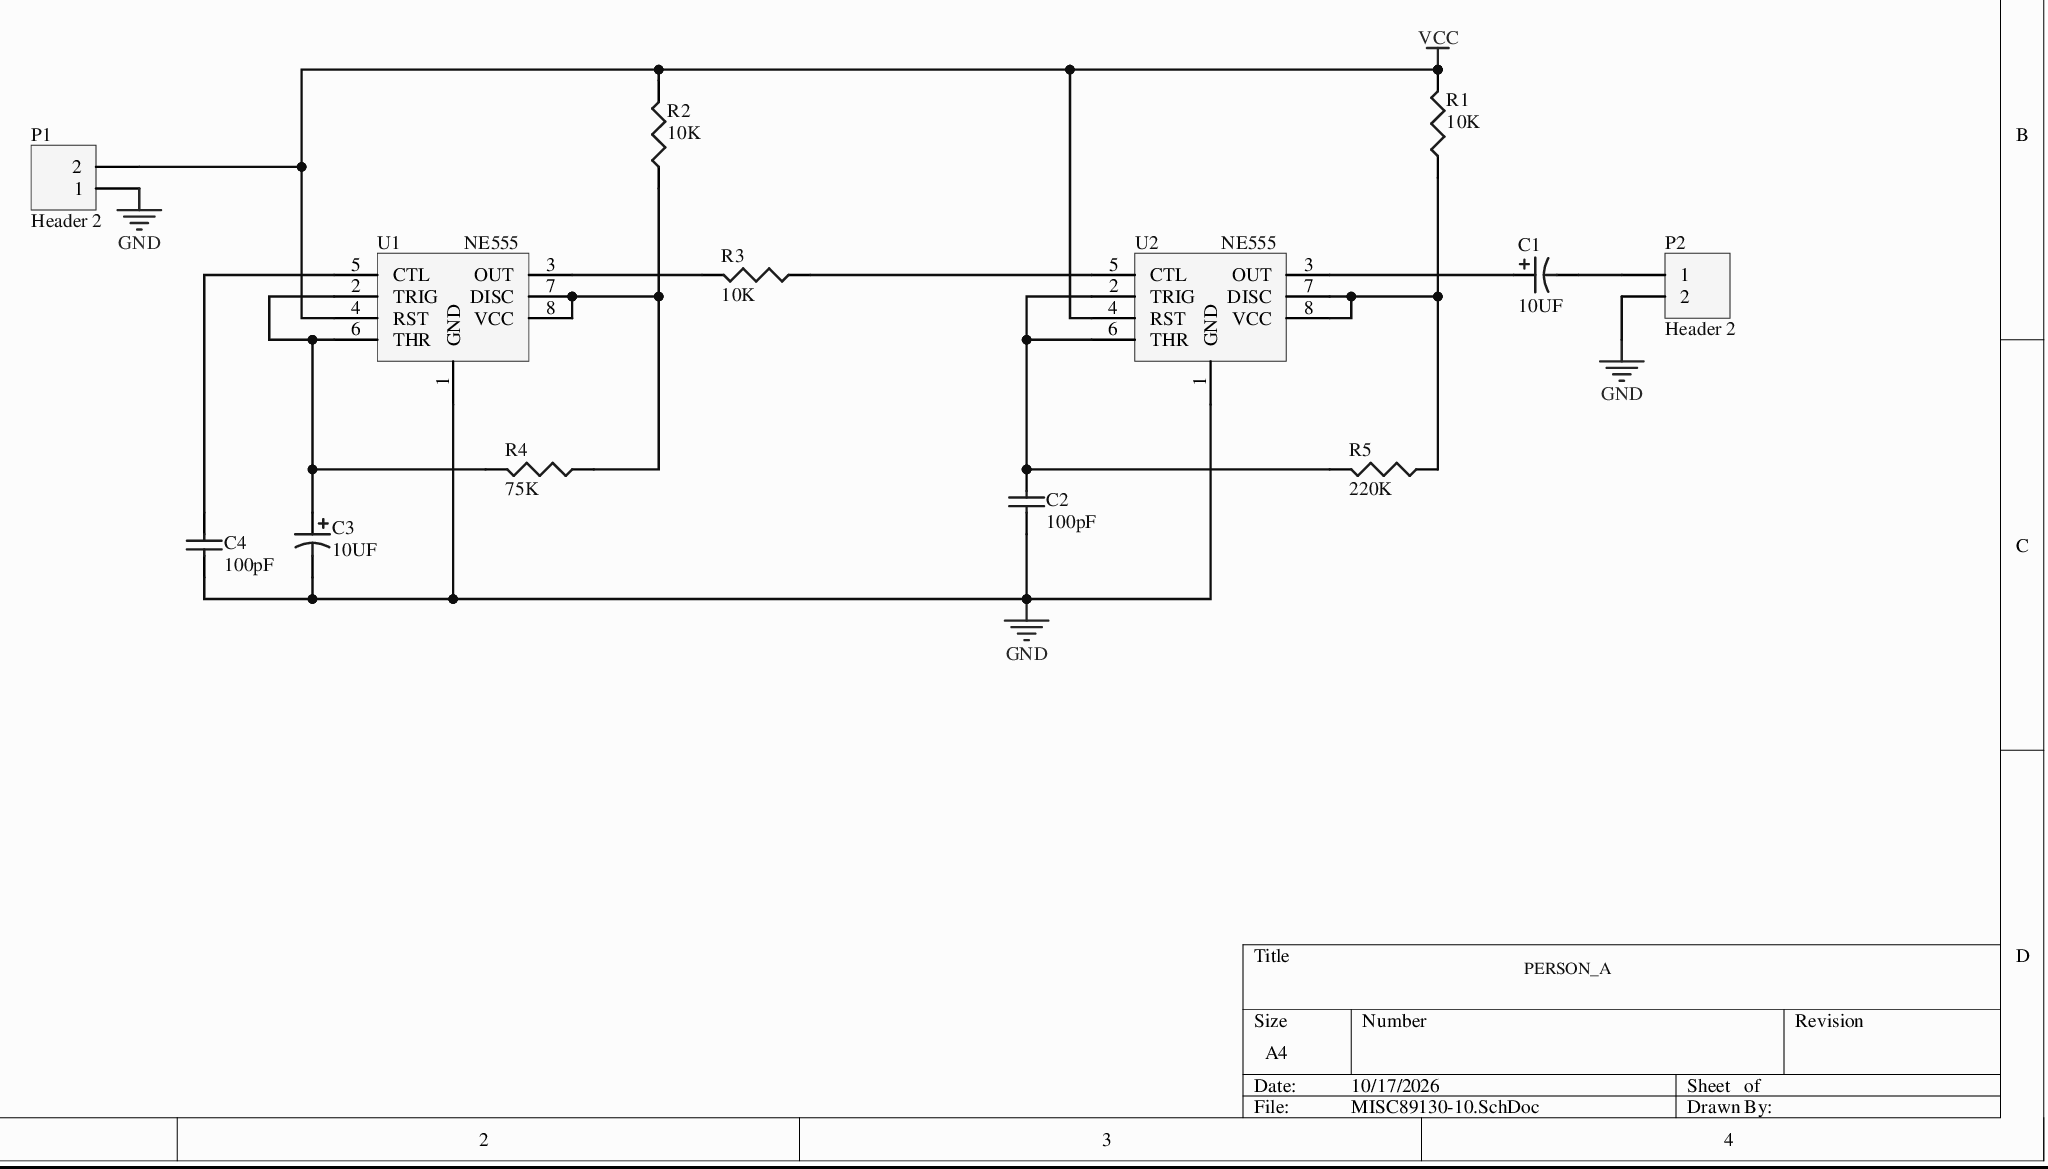
[diagram p0: MISC89130-10.SchDoc]
# Altium project MISC89130-7.PrjPcb
1 sheet, 13 parts. Net scope: global (net labels, ports and power ports of the same name join across sheets).
Board file: MISC89130.PcbDoc

## Sheet MISC89130-10.SchDoc
size A4

### Parts
C1  10UF  [C1206]
C2  value 100pF  [J1-0603]  (hidden comment: Cap)
C3  10UF  [C1206]
C4  value 100pF  [J1-0603]  (hidden comment: Cap)
P1  Header 2  [HDR1X2]
P2  Header 2  [HDR1X2]
R1  10K  [J1-0603]
R2  10K  [J1-0603]
R3  10K  [J1-0603]
R4  75K  [J1-0603]
R5  220K  [J1-0603]
U1  NE555  [DIP8]
U2  NE555  [DIP8]

### Nets
GND: C2.1 C3.2 C4.1 P1.1 P2.2 U1.1(GND) U2.1(GND)
VCC: P1.2 R1.2 R2.2 U1.4(RST) U2.4(RST)
NetC1_1: C1.1 U2.3(OUT)
NetC1_2: C1.2 P2.1
NetC2_2: C2.2 R5.2 U2.2(TRIG) U2.6(THR)
NetC3_1: C3.1 R4.2 U1.2(TRIG) U1.6(THR)
NetC4_2: C4.2 U1.5(CTL)
NetR1_1: R1.1 R5.1 U2.7(DISC) U2.8(VCC)
NetR2_1: R2.1 R4.1 U1.7(DISC) U1.8(VCC)
NetR3_1: R3.1 U2.5(CTL)
NetR3_2: R3.2 U1.3(OUT)

### Notes on the sheet
- PERSON_A

### Library data of the parts
C1 C3 = Cap Pol3: Polarized Capacitor (Surface Mount); Value: 100pF; Published: 8-Jun-2000; LatestRevisionDate: 29-May-2009; LatestRevisionNote: IPC-7351 Footprint Added.; PackageReference: C0805; PackageDescription: Chip Capacitor; Publisher: Altium Limited
C2 C4 = Cap: Capacitor; Published: 8-Jun-2000; LatestRevisionDate: 17-Jul-2002; LatestRevisionNote: Re-released for DXP Platform.; PackageReference: RAD-0.3; PackageDescription: Radial Cap, Thru-Hole; 2 Leads; 0.3 in Pin Spacing; Publisher: Altium Limited
P1 P2 = Header 2: Header, 2-Pin; LatestRevisionDate: 17-Jul-2002; LatestRevisionNote: Re-released for DXP Platform.; Publisher: Altium Limited
R1-R5 = Res3: Resistor; Value: 1K; Published: 8-Jun-2000; LatestRevisionDate: 29-May-2009; LatestRevisionNote: IPC-7351 Footprint Added.; PackageReference: J1-0603; PackageDescription: Chip Resistor; Publisher: Altium Limited